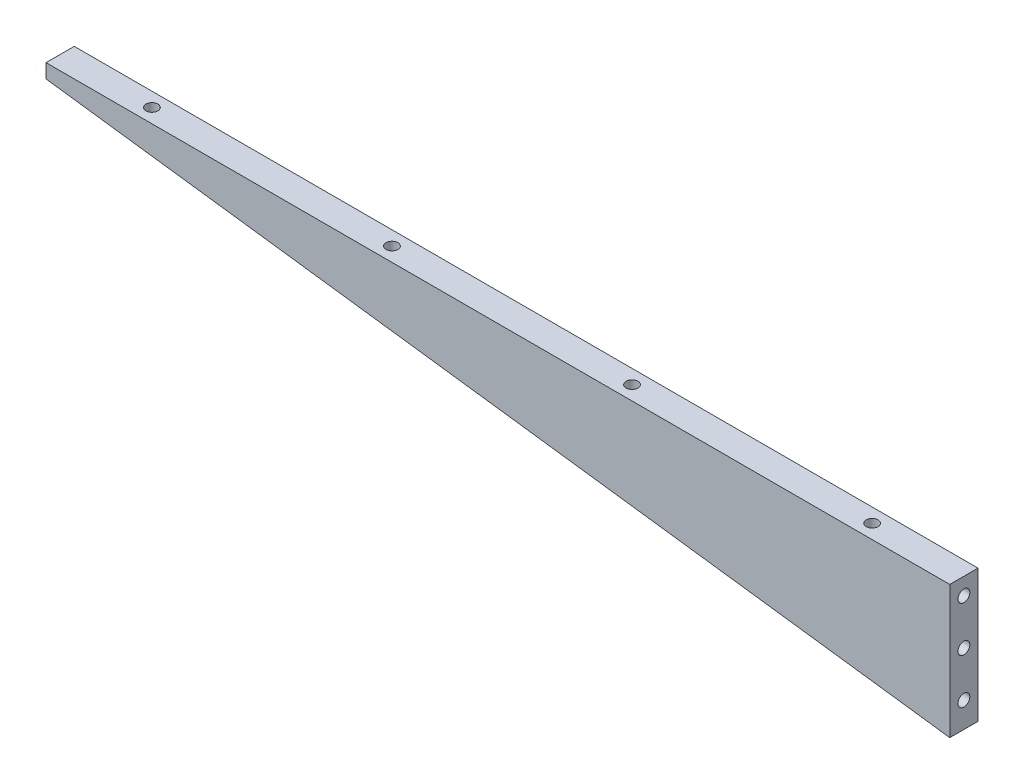
from build123d import *

# Parameters (mm, degrees)
BOSS_EXTRUDE1_DEPTH   = 10
M5_TAPPED_HOLE1_D     = 4.2
M5_TAPPED_HOLE1_DEPTH = 14
M5_TAPPED_HOLE1_TIP   = 1.2618073
M5_TAPPED_HOLE2_D     = 4.2
M5_TAPPED_HOLE2_DEPTH = 14
M5_TAPPED_HOLE2_TIP   = 1.2618073


with BuildPart() as part:
    # Sketch1 → Boss-Extrude1 (new body)
    with BuildSketch(Plane.XY):
        Polygon((0, 0), (-320, 42), (-320, 47), (0, 47), align=None)
    extrude(amount=BOSS_EXTRUDE1_DEPTH)

    # M5 Tapped Hole1
    with Locations(Plane(origin=(0, 47, 0), x_dir=(-1, 0, 0), z_dir=(0, 1, 0))):
        with Locations((287.5, 5), (202.5, 5), (117.5, 5), (32.5, 5)):
            Hole(M5_TAPPED_HOLE1_D / 2, depth=M5_TAPPED_HOLE1_DEPTH)
            with Locations((0, 0, -(M5_TAPPED_HOLE1_DEPTH + M5_TAPPED_HOLE1_TIP / 2))):  # 118° drill point
                Cone(0, M5_TAPPED_HOLE1_D / 2, M5_TAPPED_HOLE1_TIP, mode=Mode.SUBTRACT)

    # M5 Tapped Hole2
    with Locations(Plane(origin=(0, 0, 0), x_dir=(0, 0, -1), z_dir=(1, 0, 0))):
        with Locations((-5, 41), (-5, 25), (-5, 9)):
            Hole(M5_TAPPED_HOLE2_D / 2, depth=M5_TAPPED_HOLE2_DEPTH)
            with Locations((0, 0, -(M5_TAPPED_HOLE2_DEPTH + M5_TAPPED_HOLE2_TIP / 2))):  # 118° drill point
                Cone(0, M5_TAPPED_HOLE2_D / 2, M5_TAPPED_HOLE2_TIP, mode=Mode.SUBTRACT)


solid = part.part
